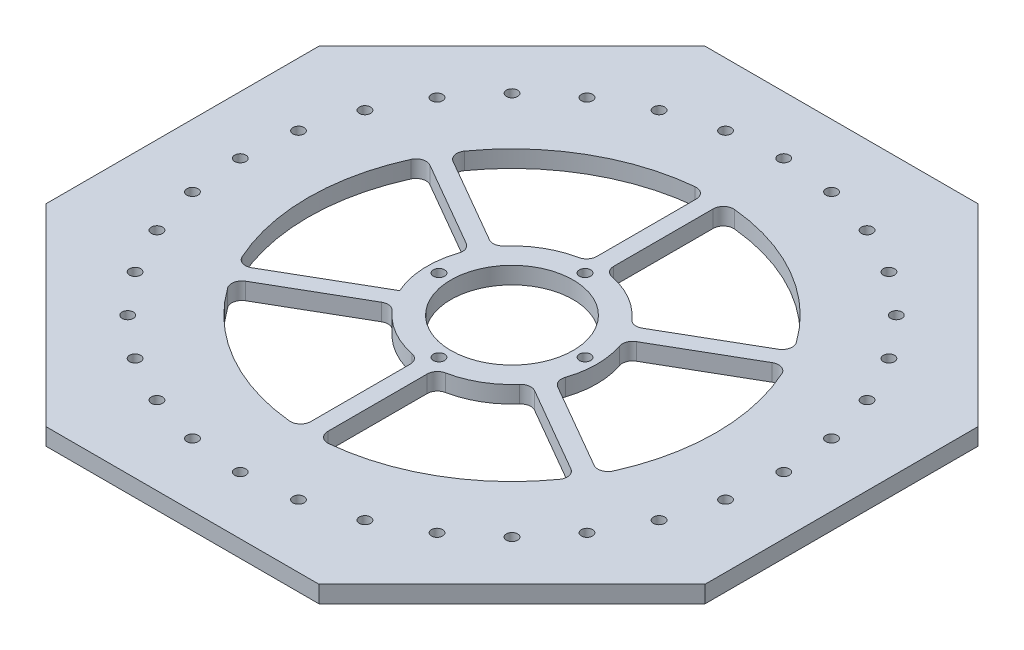
SolidWorks part; units mm, degrees
ref_plane "前视基准面" through (0, 0, 0) normal (0, 0, 1) x (1, 0, 0)
ref_plane "上视基准面" through (0, 0, 0) normal (0, 1, 0) x (1, 0, 0)
ref_plane "右视基准面" through (0, 0, 0) normal (1, 0, 0) x (0, 0, -1)
sketch "草图1" plane through (0, 0, 0) normal (0, 1, 0) x (1, 0, 0)
  line L1 (-40.1818, 97.0074) -> (-97.0074, 40.1818)
  line L2 (-97.0074, 40.1818) -> (-97.0074, -40.1818)
  line L3 (-97.0074, -40.1818) -> (-40.1818, -97.0074)
  line L4 (-40.1818, -97.0074) -> (40.1818, -97.0074)
  line L5 (40.1818, -97.0074) -> (97.0074, -40.1818)
  line L6 (97.0074, -40.1818) -> (97.0074, 40.1818)
  line L7 (97.0074, 40.1818) -> (40.1818, 97.0074)
  line L8 (40.1818, 97.0074) -> (-40.1818, 97.0074)
  circle A0 centre (0, 0) radius 18
  circle A1 centre (0, 0) radius 105 construction
  circle A2 centre (0, 0) radius 97.0074 construction
  circle A3 centre (0, 0) radius 60
  circle A4 centre (0, 0) radius 25
  dimension "D1" = 36
  dimension "D2" = 210
  dimension "D3" = 120
  dimension "D4" = 50
extrude "凸台-拉伸1" add sketch "草图1" along normal mid plane 5 contours A4 A0 | L7 L8 L1 L2 L3 L4 L5 L6 A3
sketch "草图8" plane through (0, 2.5, 0) normal (0, 1, 0) x (1, 0, 0)
  line L0 (0, 24.8747) -> (0, 0) construction
  line L1 (2.5, 24.8747) -> (-2.5, 24.8747)
  line L2 (2.5, 24.8747) -> (2.5, 64.7187)
  line L3 (2.5, 64.7187) -> (-2.5, 64.7187)
  line L4 (-2.5, 24.8747) -> (-2.5, 64.7187)
  line L5 (2.5, 24.8747) -> (-2.5, 64.7187) construction
  line L6 (2.5, 64.7187) -> (-2.5, 24.8747) construction
  circle A0 centre (0, 0) radius 25 construction
  point P0 (0, 44.7967)
  dimension "D1" = 5
extrude "凸台-拉伸2" add sketch "草图8" against normal up to surface (5 mm away) up to face at (0, -2.5, 60)
pattern_circular "阵列(圆周)3" count 6 over 360 about axis through (0, 0, 0) along (0, 1, 0) of "凸台-拉伸2"
sketch "草图9" plane through (0, 2.5, 0) normal (0, 1, 0) x (1, 0, 0)
  circle A0 centre (0, 0) radius 25
  arc A1 (20.2921, 14.6024) -> (2.5, 24.8747) centre (0, 0) ccw construction
  circle A2 centre (0, 0) radius 18 construction
  circle A3 centre (0, 0) radius 18
extrude "凸台-拉伸3" add sketch "草图9" along normal blind 12
sketch "草图11" plane through (0, 2.5, 0) normal (0, 1, 0) x (1, 0, 0)
  line L0 (0, 0) -> (0, 80) construction
  circle A0 centre (0, 80) radius 1.65
  dimension "D1" = 3.3
  dimension "D2" = 80
extrude "切除-拉伸3" cut sketch "草图11" against normal blind 8
pattern_circular "阵列(圆周)5" count 32 over 360 about axis through (0, 0, 0) along (0, 1, 0) of "切除-拉伸3"
sketch "草图12" plane through (0, 0, 0) normal (0, 0, 1) x (1, 0, 0)
  line L0 (0, 14.5) -> (0, 9.5) construction
  line L1 (25, 14.5) -> (-25, 14.5) construction
  circle A0 centre (0, 9.5) radius 2.2
  dimension "D1" = 5
  dimension "D2" = 4.4
extrude "切除-拉伸4" cut sketch "草图12" against normal blind 45
sketch "草图13" plane through (0, 0, 0) normal (0, 0, 1) x (1, 0, 0)
  circle A0 centre (0, 9.5) radius 4
  dimension "D1" = 8
extrude "切除-拉伸5" cut sketch "草图13" against normal blind 45 from offset 24 offset against normal yes
pattern_circular "阵列(圆周)6" count 4 over 360 about axis through (0, 0, 0) along (0, 1, 0) of "切除-拉伸4", "切除-拉伸5"
sketch "草图14" plane through (0, 14.5, 0) normal (0, 1, 0) x (1, 0, 0)
  circle A1 centre (0, 0) radius 25
  circle A2 centre (0, 0) radius 25
  dimension "D1" = 0
extrude "切除-拉伸6" cut sketch "草图14" against normal up to surface (12 mm away) up to face at (29.9832, 2.5, -72.386)
fillet "圆角1" radius 3 23 edges at (-2.5, 0, 59.9479) (2.5, 0, 59.9479) (20.2921, 0, 14.6024) (2.5, 0, 24.8747) (-2.5, 0, 24.8747) (50.6664, 0, 32.139) (53.1664, 0, 27.8089) (53.1664, 0, -27.8089) (22.7921, 0, -10.2723) (22.7921, 0, 10.2723) (20.2921, 0, -14.6024) (50.6664, 0, -32.139) (2.5, 0, -24.8747) (2.5, 0, -59.9479) (-20.2921, 0, -14.6024) (-2.5, 0, -24.8747) (-2.5, 0, -59.9479) (-50.6664, 0, -32.139) (-53.1664, 0, -27.8089) (-22.7921, 0, -10.2723) (-20.2921, 0, 14.6024) (-50.6664, 0, 32.139) (-53.1664, 0, 27.8089)
sketch "草图15" plane through (0, 2.5, 0) normal (0, 1, 0) x (1, 0, 0)
  line L0 (0, 0) -> (0, 21.5) construction
  circle A0 centre (0, 21.5) radius 1.65
  dimension "D1" = 3.3
  dimension "D2" = 21.5
extrude "切除-拉伸7" cut sketch "草图15" against normal blind 10
pattern_circular "阵列(圆周)7" count 4 over 360 about axis through (0, 0, 0) along (0, 1, 0) of "切除-拉伸7"
